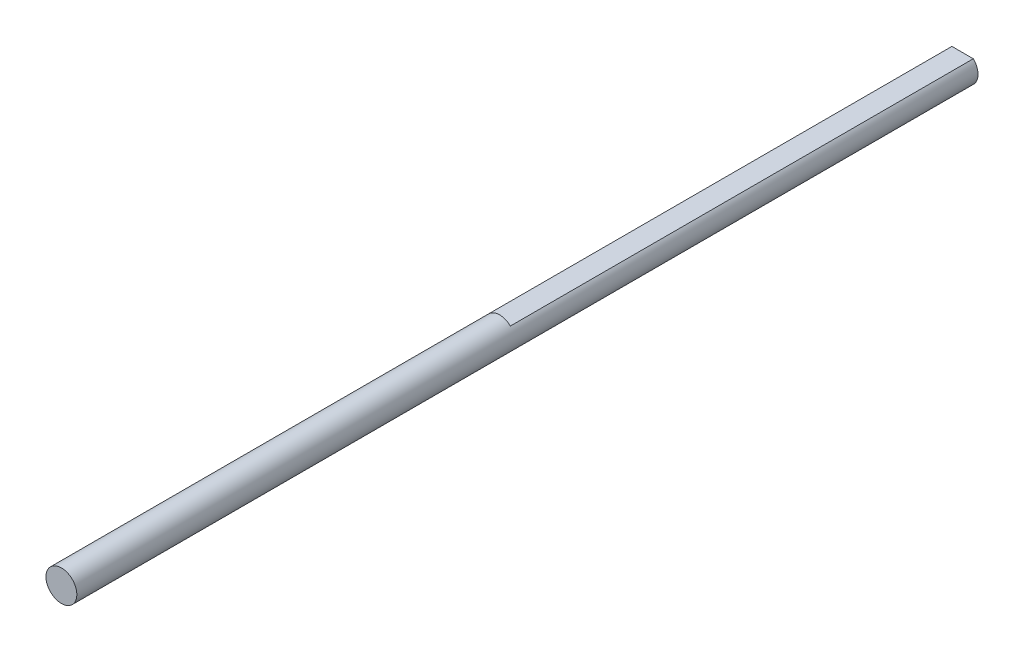
from build123d import *

# Parameters (mm, degrees)
SKETCH1_R           = 2.5
BOSS_EXTRUDE1_DEPTH = 162
CUT_EXTRUDE1_DEPTH  = 75
CUT_EXTRUDE2_START  = -16
SKETCH3_R           = 2.5
CUT_EXTRUDE2_DEPTH  = 16


with BuildPart() as part:
    # Sketch1 → Boss-Extrude1 (new body)
    with BuildSketch(Plane.XY):
        Circle(SKETCH1_R)
    extrude(amount=BOSS_EXTRUDE1_DEPTH)

    # Sketch2 → Cut-Extrude1 (cut)
    with BuildSketch(Plane(origin=(0, 0, 0), x_dir=(-1, 0, 0), z_dir=(0, 0, -1))):
        with BuildLine():
            Line((0, 1.8), (1.734935157, 1.8))
            ThreePointArc((1.734935157, 1.8), (0, 2.5), (-1.734935157, 1.8))
            Line((-1.734935157, 1.8), (0, 1.8))
        make_face()
    extrude(amount=-CUT_EXTRUDE1_DEPTH, mode=Mode.SUBTRACT)

    # Sketch3 → Cut-Extrude2 (cut)
    with BuildSketch(Plane.XY.offset(162).offset(CUT_EXTRUDE2_START)):
        with Locations(Location((0, 0, 0), (0, 0, 133.945519562))):
            Circle(SKETCH3_R)
    extrude(amount=CUT_EXTRUDE2_DEPTH, mode=Mode.SUBTRACT)


solid = part.part
